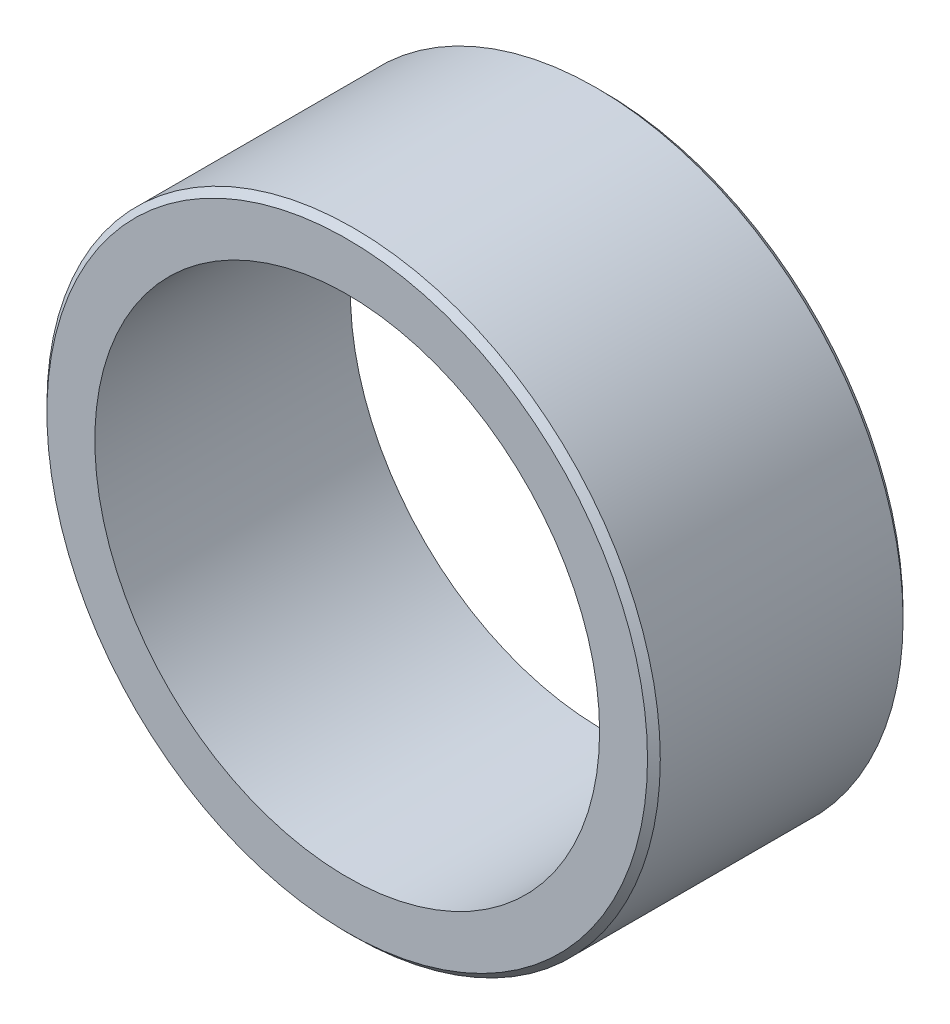
from build123d import *

# Parameters (mm, degrees)
SKETCH1_R           = 24
SKETCH1_R_2         = 19.75
BOSS_EXTRUDE1_DEPTH = 10
CHAMFER1_SIZE       = 0.5


with BuildPart() as part:
    # Sketch1 → Boss-Extrude1 (new, symmetric)
    with BuildSketch(Plane.XY):
        Circle(SKETCH1_R)
        Circle(SKETCH1_R_2, mode=Mode.SUBTRACT)
    extrude(amount=BOSS_EXTRUDE1_DEPTH, both=True)

    # Chamfer1
    chamfer1_edges = [part.edges().sort_by_distance(p)[0] for p in [
        (-24, 0, -10),
        (-24, 0, 10),
    ]]
    chamfer(chamfer1_edges, length=CHAMFER1_SIZE)


solid = part.part
